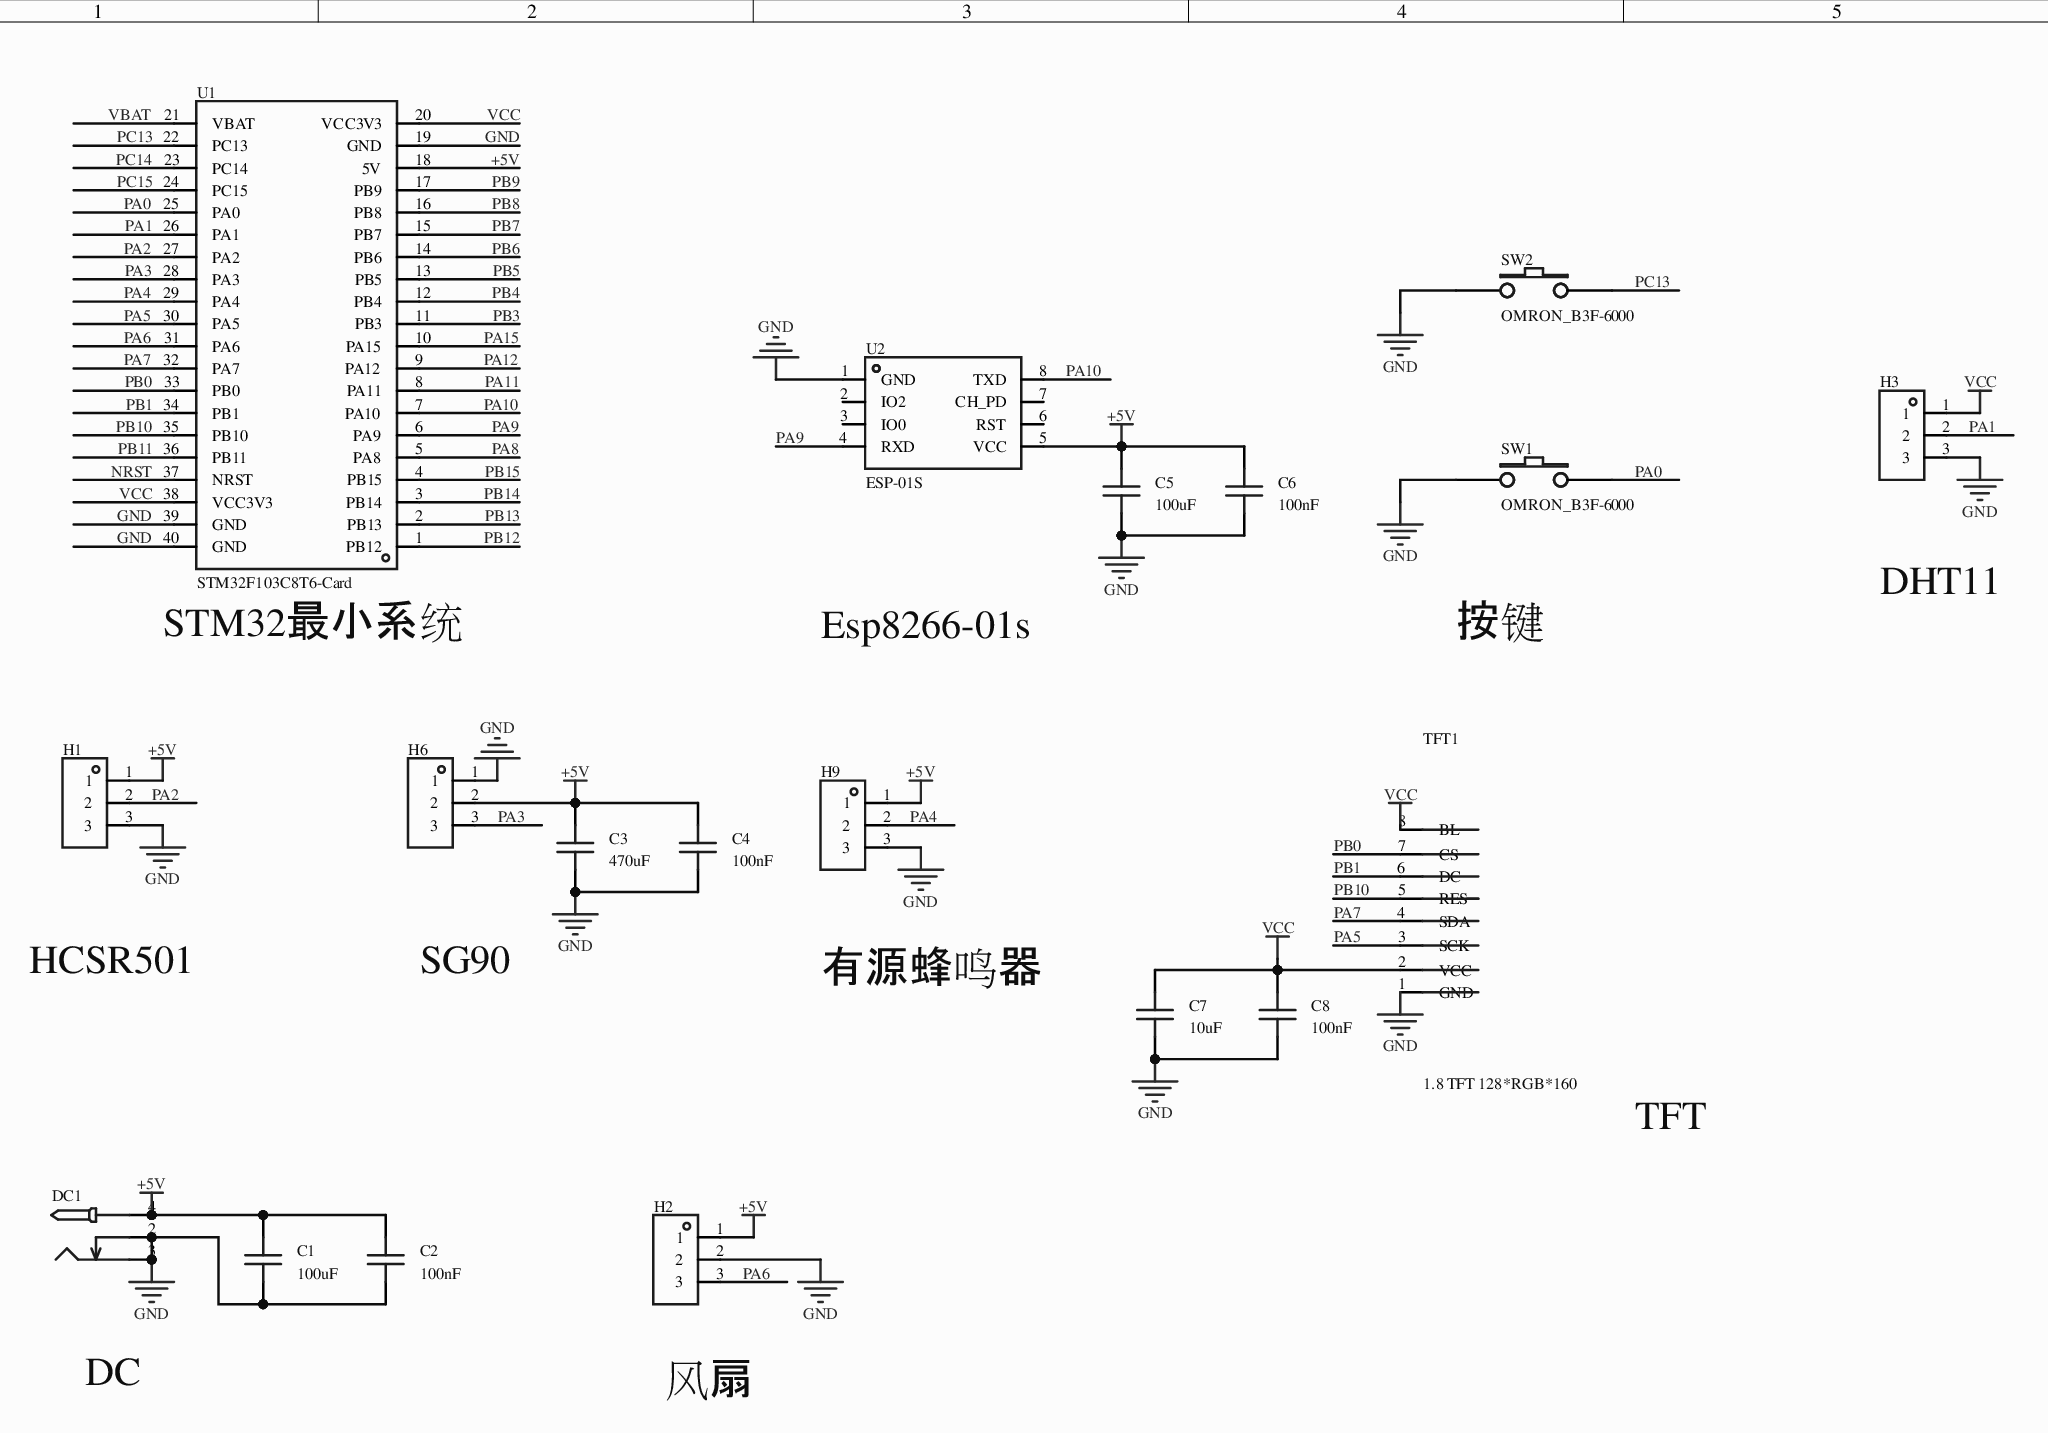
[diagram p0: MISC52046-3.schdoc]
# Altium project MISC52046-2.PrjPcb
1 sheet, 19 parts. Net scope: global (net labels, ports and power ports of the same name join across sheets).
Board file: MISC52046.pcbdoc

## Sheet MISC52046-3.schdoc
size 297 x 209 mm; Version: V1.0; @Project Name: MISC52046; @Page Count: 1; @Update Date: 2026-05-06; @Create Date: 2026-05-06; @Schematic Name: MISC52046; @Page No: 1; @Create Time: 23:22:16; @Update Time: 17:32:40; @Board Name: MISC52046

### Parts
C1  100uF  [C0805]
C2  100nF  [C0805]
C3  470uF  [C0805]
C4  100nF  [C0805]
C5  100uF  [C0805]
C6  100nF  [C0805]
C7  10uF  [C0805]
C8  100nF  [C0805]
DC1  (no value)  [DC-2.0]
H1  (no value)  [HDR-TH_3P-P2.54-V-F]
H2  (no value)  [HDR-TH_3P-P2.54-V-F]
H3  (no value)  [HDR-TH_3P-P2.54-V-F]
H6  (no value)  [HDR-TH_3P-P2.54-V-F]
H9  (no value)  [HDR-TH_3P-P2.54-V-F]
SW1  OMRON_B3F-6000  [KEY-TH_2P-L6.0-W6.0-P5.00]
SW2  OMRON_B3F-6000  [KEY-TH_2P-L6.0-W6.0-P5.00]
TFT1  1.8 TFT 128*RGB*160  [LCD-TH_8P-P2.54-L56.0-W34.0_1.8-TFT]
U1  STM32F103C8T6-Card  [CONN-TH_L53.3-W22.9_STM32F103C8T6-CARD]
U2  ESP-01S  [WIFIM-TH_ESP-01S]

### Nets
+5V: C1.2 C2.2 C3.2 C4.2 C5.2 C6.2 DC1.4 H1.1 H2.1 H6.2 H9.1 U1.18(5V) U2.5(VCC)
GND: C1.1 C2.1 C3.1 C4.1 C5.1 C6.1 C7.1 C8.1 DC1.2 DC1.3 H1.3 H2.2 H3.3 H6.1 H9.3 SW1.1 SW2.1 TFT1.1(GND) U1.19(GND) U1.39(GND) U1.40(GND) U2.1(GND)
VCC: C7.2 C8.2 H3.1 TFT1.2(VCC) TFT1.8(BL) U1.20(VCC3V3) U1.38(VCC3V3)
NRST: U1.37(NRST)
PA0: SW1.2 U1.25(PA0)
PA1: H3.2 U1.26(PA1)
PA2: H1.2 U1.27(PA2)
PA3: H6.3 U1.28(PA3)
PA4: H9.2 U1.29(PA4)
PA5: TFT1.3(SCK) U1.30(PA5)
PA6: H2.3 U1.31(PA6)
PA7: TFT1.4(SDA) U1.32(PA7)
PA8: U1.5(PA8)
PA9: U1.6(PA9) U2.4(RXD)
PA10: U1.7(PA10) U2.8(TXD)
PA11: U1.8(PA11)
PA12: U1.9(PA12)
PA15: U1.10(PA15)
PB0: TFT1.7(CS) U1.33(PB0)
PB1: TFT1.6(DC) U1.34(PB1)
PB3: U1.11(PB3)
PB4: U1.12(PB4)
PB5: U1.13(PB5)
PB6: U1.14(PB6)
PB7: U1.15(PB7)
PB8: U1.16(PB8)
PB9: U1.17(PB9)
PB10: TFT1.5(RES) U1.35(PB10)
PB11: U1.36(PB11)
PB12: U1.1(PB12)
PB13: U1.2(PB13)
PB14: U1.3(PB14)
PB15: U1.4(PB15)
PC13: SW2.2 U1.22(PC13)
PC14: U1.23(PC14)
PC15: U1.24(PC15)
VBAT: U1.21(VBAT)

Not connected (* = marked no-connect by the designer): U2 2(IO2)* 3(IO0)* 6(RST)* 7(CH_PD)*

### Notes on the sheet
- (near U1) STM32最小系统
- Esp8266-01s
- 按键
- DHT11
- HCSR501
- SG90
- 有源蜂鸣器
- TFT
- DC
- (near H2) 风扇

### Library data of the parts
C1-C8 = CAP_0805: Symbol: Capacitance; ConvertToPcb: yes; ModelId: 1ba041120af144c991958decab20d2410819f05c4eef4c71ace90d822a990e87; ModelName: C0805_L2.0-W1.3-H1.3; ModelTransform: 78.74,51.181,0,0,0,0,0,0.0005,0; Device: CAP_0805; AddInBom: yes; Supplier Footprint: 0805; FootprintName: C0805
  C1 C5: Value: 100uF
  C2 C4 C6 C8: Value: 100nF
  C3: Value: 470uF
  C7: Value: 10uF
DC1 = DC-005_2.0: Symbol: DC电源接口; ConvertToPcb: yes; ModelId: f5f20b8a2308479b936ba3c2698865bb0819f05c4eef4c71ace90d822a990e87; ModelName: DC-IN-TH_DC-5520-1; ModelTransform: 372.05,551.18,582.68,90,0,0,137.8,0,-149.61; Device: DC-005_2.0; AddInBom: yes; Supplier Footprint: 插件; FootprintName: DC-2.0
H1-H3 H6 H9 = HDR-F_2.54_1x3P: Symbol: PM254V-11-03-H85; 3D Model: f3b3cc5aae9641bf9e56fc160cef875b; 3D Model Transform: 299.9994,100,0,0,0,0,0,0,-118.11; ConvertToPcb: yes; ModelName: HDR2.54-F-LI-1X3P; Device: HDR-F_2.54_1x3P; Supplier Part: C541850; Supplier Footprint: 插件; FootprintName: HDR-TH_3P-P2.54-V-F; AddInBom: yes
SW1 SW2 = OMRON_B3F-6000: AddInBom: yes; ModelId: d13ad252cbf84dc495704a853cd2bab60819f05c4eef4c71ace90d822a990e87; ModelName: KEY-TH_2P-L6.0-W6.0-H5.0-P5.00; ModelTransform: 236.22,236.22,0,0,0,0,0,0,-137.795; Symbol: OMRON_B3F-6000; Device: OMRON_B3F-6000; LCSC Part Name: OMRON_B3F-6000; SupplierPart: C9900006128; ManufacturerPart: OMRON_B3F-6000; Supplier Footprint: SWITCH6*6*4.3; JLCPCB Part Class: Extended Part; Supplier: LCSC; ConvertToPcb: yes; FootprintName: KEY-TH_2P-L6.0-W6.0-P5.00
TFT1 = 1.8 TFT 128*RGB*160: AddInBom: yes; Symbol: 1.8 TFT 128*RGB*160; Device: 1.8 TFT 128*RGB*160; LCSC Part Name: 1.8 TFT 128*RGB*160; SupplierPart: C9900080251; ManufacturerPart: 1.8 TFT 128*RGB*160; Supplier Footprint: 插件; Supplier: LCSC; ConvertToPcb: yes; FootprintName: LCD-TH_8P-P2.54-L56.0-W34.0_1.8-TFT
U1 = STM32F103C8T6-Card: AddInBom: yes; Device: STM32F103C8T6-Card; Symbol: STM32F103C8T6-CARD; FootprintName: CONN-TH_L53.3-W22.9_STM32F103C8T6-CARD; LCSC Part Name: STM32F103C8T6-Card; SupplierPart: C9900077949; ManufacturerPart: STM32F103C8T6-Card; Supplier Footprint: 插件; Supplier: LCSC; ConvertToPcb: yes
U2 = ESP-01S_C111009: 3D Model: eb7175da78ae48b3b1568cfe3027405f0819f05c4eef4c71ace90d822a990e87; 3D Model Transform: 582.676,976.37608,0,0,0,0,0,388.346,-118.11; AddInBom: yes; Symbol: ESP-01S; Device: ESP-01S_C111009; LCSC Part Name: ESP-01S; Supplier Part: C111009; Manufacturer Part: ESP-01S; Supplier Footprint: -; JLCPCB Part Class: Extended Part; Supplier: LCSC; ConvertToPcb: yes; FootprintName: WIFIM-TH_ESP-01S; ModelName: WIFIM-TH_ESP-01S